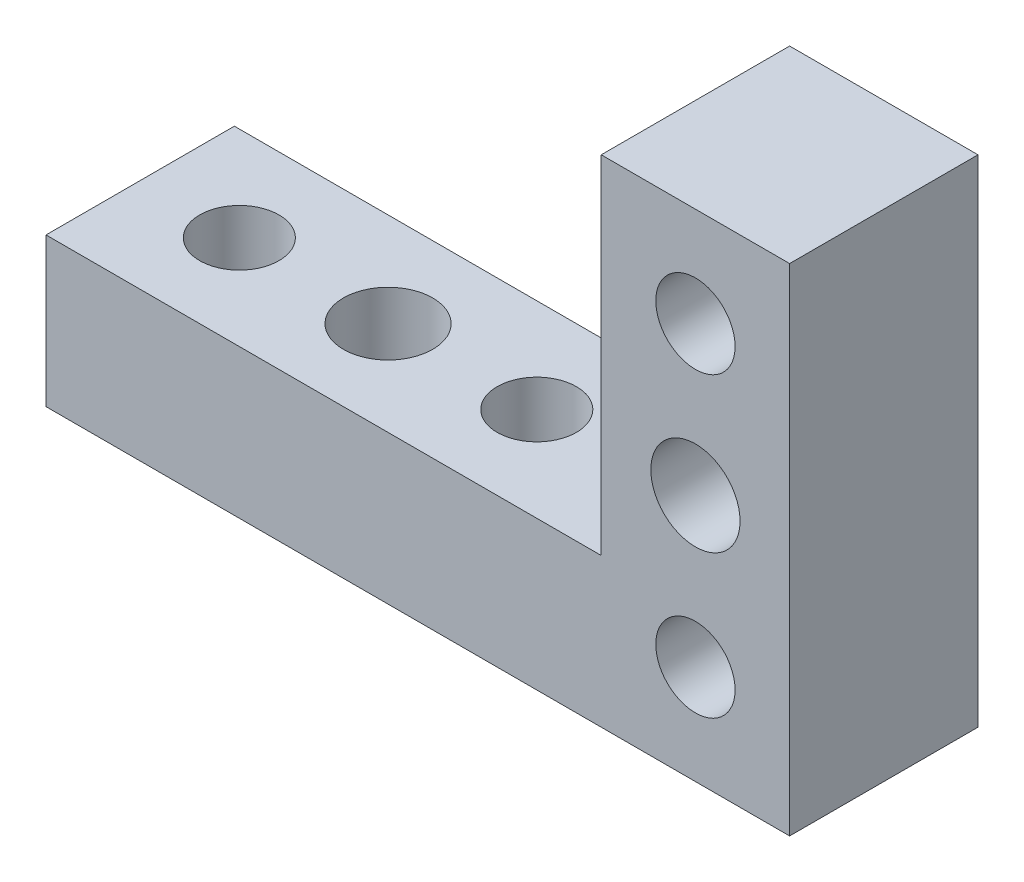
SolidWorks part; units mm, degrees
ref_plane "Front Plane" through (0, 0, 0) normal (0, 0, 1) x (1, 0, 0)
ref_plane "Top Plane" through (0, 0, 0) normal (0, 1, 0) x (1, 0, 0)
ref_plane "Right Plane" through (0, 0, 0) normal (1, 0, 0) x (0, 0, -1)
sketch "Sketch1" plane through (0, 0, 0) normal (0, 0, 1) x (1, 0, 0)
  line L0 (0, 0) -> (75, 0)
  line L1 (75, 0) -> (75, 50)
  line L2 (75, 50) -> (56, 50)
  line L3 (56, 50) -> (56, 15)
  line L4 (56, 15) -> (0, 15)
  line L5 (0, 15) -> (0, 0)
  line L6 (65.5, 50) -> (65.5, 0) construction
  circle A0 centre (65.5, 10) radius 4
  circle A1 centre (65.5, 25) radius 4.5
  circle A2 centre (65.5, 40) radius 4
  dimension "D5" = 10
  dimension "D6" = 15
  dimension "D7" = 15
  dimension "D1" = 75
  dimension "D2" = 15
  dimension "D3" = 56
  dimension "D4" = 35
extrude "Boss-Extrude1" add sketch "Sketch1" along normal blind 19
ref_plane "Plane1" through (0, 15, 0) normal (0, 1, 0) x (1, 0, 0)
sketch "Sketch2" plane through (0, 15, 0) normal (0, 1, 0) x (1, 0, 0)
  line L0 (0, -9.5) -> (56, -9.5) construction
  line L1 (0, -19) -> (0, 0) construction
  line L2 (56, -19) -> (56, 0) construction
  circle A0 centre (10, -9.5) radius 4
  circle A1 centre (25, -9.5) radius 4.5
  circle A2 centre (40, -9.5) radius 4
  dimension "D1" = 10
  dimension "D2" = 8
  dimension "D3" = 15
  dimension "D4" = 15
  dimension "D5" = 9
  dimension "D6" = 8
extrude "Cut-Extrude1" cut sketch "Sketch2" against normal blind 19
